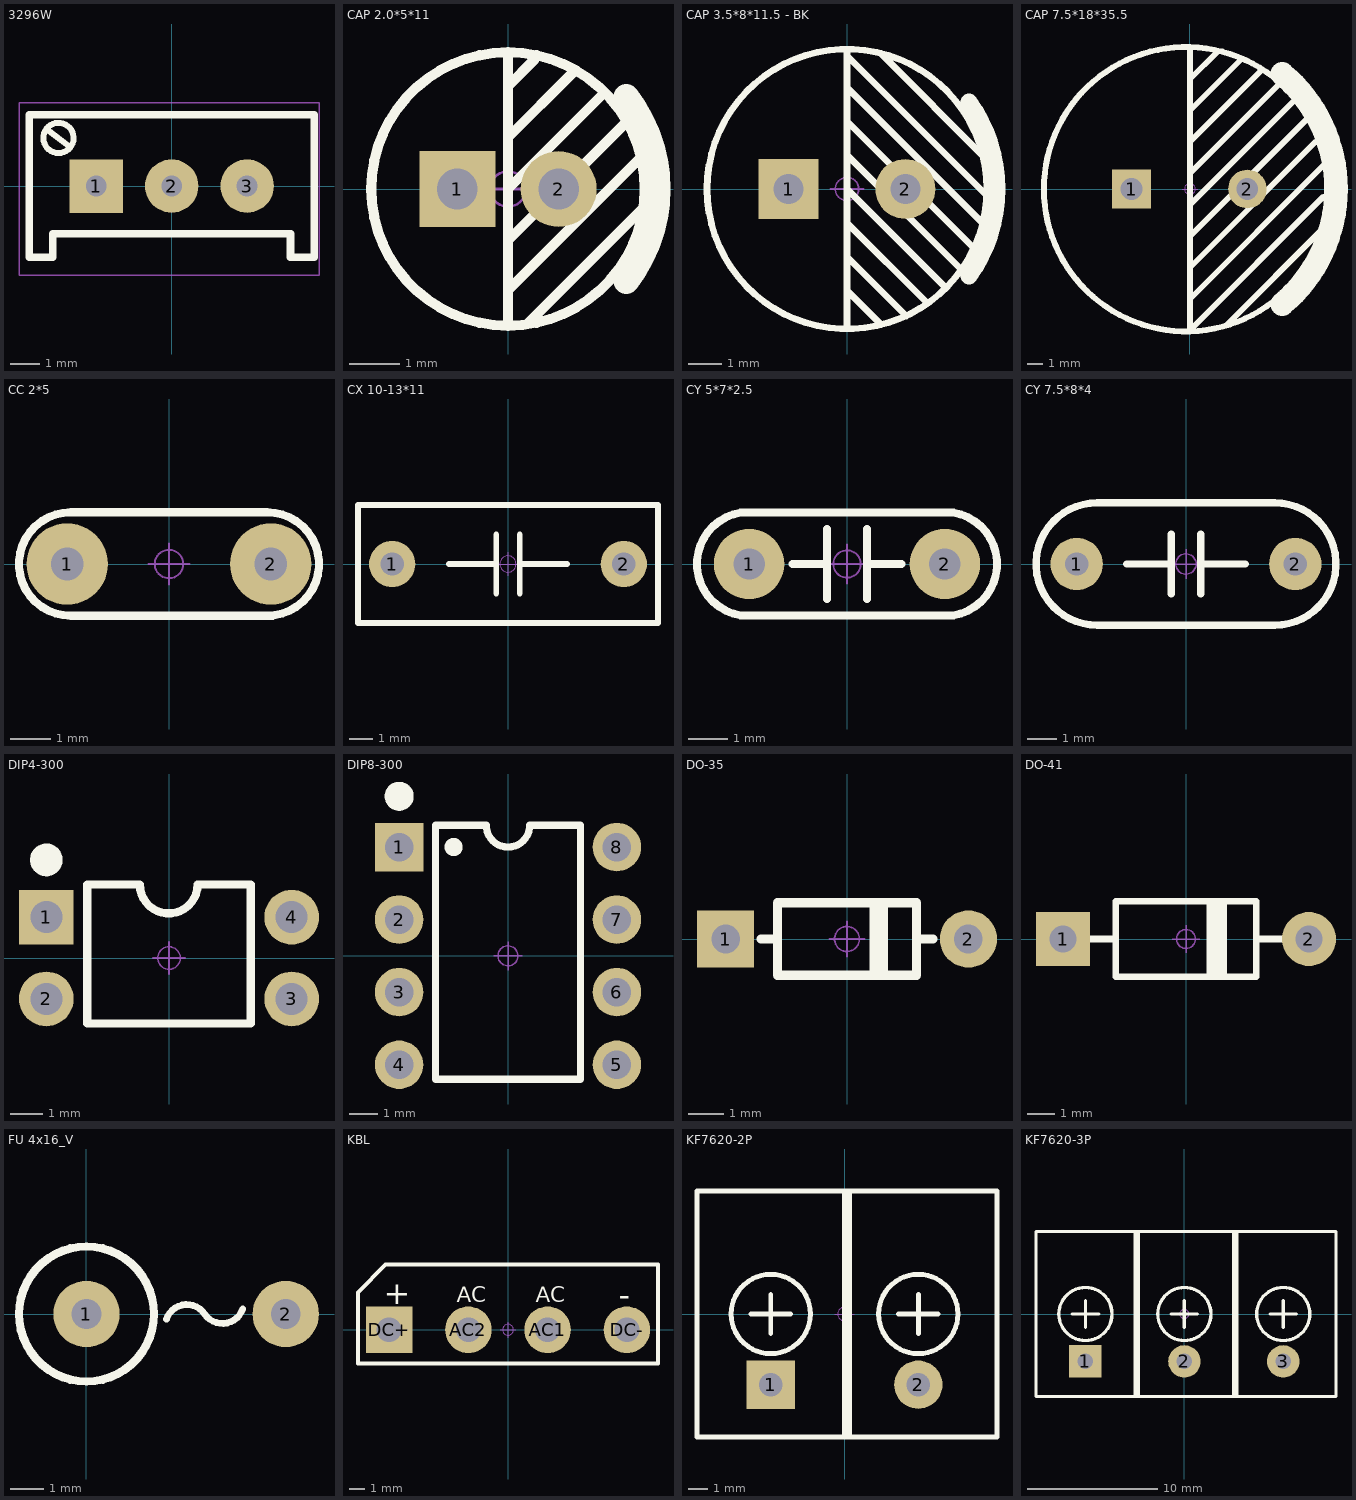
[diagram p0: the footprints below, top view; thin cyan lines are the x and y axes]
# Altium footprint library MISC82119-3.PcbLib: 27 footprints (part 1 of 2)
Each footprint in its own frame and in the unit in brackets; x right, y up, seen from the top. Pads: shape width x height; smd on the part's side, far side on the other; paste and mask are expansions set on the pad; w line width, h text height; cw(c..) or ccw(c..) is an arc to the next point about the centre after c.

## 3296W [mm] "Precise Multi-Winding Adjustable Resistor"
height 6.35
pads (3):
  rect 1.8x1.8 hole 0.7: 1(-2.54,0)
  round 1.8 hole 0.7: 2(0,0) 3(2.54,0)
Top Overlay:
  lines w0.2: -3.302,1.651 ccw(c-3.81,1.618) -3.301,1.608
  lines w0.203: -4.2,1.9 -3.464,1.348
  lines w0.254: -4.8,-2.4 -4,-2.4 -4,-1.6 4,-1.6 4,-2.4 4.8,-2.4 4.8,2.4 -4.8,2.4 -4.8,-2.4
Mechanical 15:
  lines w0.05: -5.14,-3 -5.14,2.8 4.96,2.8 4.96,-3 -5.14,-3
3D body "3296.STEP": height 11.52, standoff -3.48, extent -4.75,-2.4 4.75,2.4

## CAP 2.0*5*11 [mm]
pads (2):
  rect 1.5x1.5 hole 0.8: 1(-1,0)
  round 1.5 hole 0.8: 2(1,0)
Top Overlay:
  circle w0.2: c0,0 r2.7
  lines w0.2: 0,-2.667 0,-2 ; 0,-1.016 2.286,1.27 ; 0,0 1.905,1.905 ; 0,1.016 1.27,2.286 ; 0,2.032 0.508,2.54 ; 0,2.667 0,-2 ; 0.381,-2.667 2.667,-0.381 ; 2.651,0.651 0,-2
  lines w0.5: 2.338,-1.819 ccw(c0,0) 2.338,1.819
Mechanical 15:
  circle w0.05: c0,0 r0.35
  lines w0.05: -0.5,0 0.5,0 ; 0,-0.5 0,0.5
3D body "CAP 2X5X11.STEP": height 11.04, standoff -3.42, extent -2.5,-2.499 2.51,2.499

## CAP 3.5*8*11.5 - BK [mm] "Pin pitch 3.5mm, diameter 8mm, height 11.5mm"
pads (2):
  rect 1.8x1.8 hole 0.9: 1(-1.75,0)
  round 1.8 hole 0.9: 2(1.75,0)
Top Overlay:
  circle w0.2: c0,0 r4.2
  lines w0.2: 0,-4.191 0,4 ; 0,-3.048 1.016,-4.064 ; 0,-2.032 1.778,-3.81 ; 0,-1.016 2.413,-3.429 ; 0,0 2.921,-2.921 ; 0,1.016 3.429,-2.413 ; 0,2.032 3.81,-1.778 ; 0,3.048 4.064,-1.016 ; 0,4.191 0,4 ; 1.016,4.064 4.191,0.889 ; 4.191,-0.127 4.127,-0.127 0,4
  lines w0.504: 3.663,-2.616 ccw(c0,0) 3.663,2.616
Mechanical 15:
  circle w0.05: c0,0 r0.35
  lines w0.05: -0.5,0 0.5,0 ; 0,-0.5 0,0.5
3D body "CAP 3.5X8X11.5.STEP": height 11.54, standoff -3.37, extent -4,-4 4.01,4

## CAP 7.5*18*35.5 [mm]
height 6.35
pads (2):
  rect 2.5x2.5 hole 1.4: 1(-3.78,0)
  round 2.5 hole 1.4: 2(3.72,0)
Top Overlay:
  circle w0.381: c-0.248,-0.013 r9.2
  lines w0.381: 0,-7.112 8.636,1.524 ; 0,-5.08 8.128,3.048 ; 0,-3.048 7.62,4.572 ; 0,-1.016 6.731,5.715 ; 0,1.016 5.715,6.731 ; 0,3.048 4.572,7.62 ; 0,5.08 3.302,8.382 ; 0,7.112 1.778,8.89 ; 0,9.144 0,-9.144 8.636,-0.508 ; 2.413,-8.763 8.636,-2.54
  lines w1.524: 5.959,-7.456 ccw(c-0.254,0) 5.959,7.456
Mechanical 15:
  circle w0.05: c0,0 r0.35
  lines w0.05: -0.5,0 0.5,0 ; 0,-0.5 0,0.5
3D body "CAP 7.5X18X35.5.STEP": height 35.54, standoff -3.37, extent -9,-8.997 9.01,8.997

## CC 2*5 [mm] "Pin pitch 2.2mm, diameter 5mm"
height 6.35
pads (2):
  round 2 hole 0.8: 1(-2.5,0) 2(2.5,0)
Top Overlay:
  lines w0.2: -2.413,1.27 2.413,1.27 ; -2.413,1.271 ccw(c-2.413,0.001) -2.413,-1.27 2.54,-1.27 ; 2.413,-1.27 ccw(c2.413,0.001) 2.413,1.271
Mechanical 15:
  circle w0.05: c0,0 r0.35
  lines w0.05: -0.5,0 0.5,0 ; 0,-0.5 0,0.5
3D body "CC 2.2X5.STEP": height 4.8, standoff -3.5, extent -2.4,-0.917 2.4,0.918

## CX 10-13*11 [mm]
pads (2):
  round 2 hole 1: 1(-5,0) 2(5,0)
Top Overlay:
  lines w0.254: -2.54,0 -0.604,0 ; -0.508,-1.27 -0.508,1.27 ; 0.508,-1.27 0.508,1.27 ; 0.508,0 2.54,0 ; -6.477,-2.54 4.953,-2.54 6.477,-2.54 6.477,2.54 4.953,2.54 -6.477,2.54 -6.477,-2.54
Mechanical 15:
  circle w0.05: c0,0 r0.35
  lines w0.05: -0.5,0 0.5,0 ; 0,-0.5 0,0.5
3D body "CX 10X13X11.STEP": height 11.02, standoff -3.48, extent -6.5,-2.5 6.5,2.5

## CY 5*7*2.5 [mm]
pads (2):
  round 1.8 hole 0.8: 1(-2.5,0) 2(2.5,0)
Top Overlay:
  lines w0.203: -1.397,0 -0.508,0 ; -0.508,-0.889 -0.508,0.889 ; 0.508,-0.889 0.508,0.889 ; 0.508,0 1.397,0 ; -2.726,1.313 ccw(c-2.5,0) -2.726,-1.313 2.726,-1.313 2.726,-1.313 ccw(c2.5,0) 2.726,1.313 -2.726,1.313 -2.726,1.313
Mechanical 15:
  circle w0.05: c0,0 r0.35
  lines w0.05: -0.5,0 0.5,0 ; 0,-0.5 0,0.5
3D body "CY 5X7X2.5.STEP": height 7, standoff -3.5, extent -3.5,-1.25 3.5,1.25

## CY 7.5*8*4 [mm] "Pin pitch 7.5mm, diameter 8mm, thickness 4mm"
height 6.35
pads (2):
  round 1.8 hole 0.8: 1(-3.75,0) 2(3.75,0)
Top Overlay:
  lines w0.254: -2.032,0 -0.508,0 ; -0.508,-1.016 -0.508,1.016 ; 0.508,-1.016 0.508,1.016 ; 0.508,0 2.032,0 ; -3.048,-2.1 cw(c-3.048,0) -3.048,2.1 3.048,2.1 cw(c3.048,0) 3.048,-2.1 -3.048,-2.1
Mechanical 15:
  circle w0.05: c0,0 r0.35
  lines w0.05: -0.5,0 0.5,0 ; 0,-0.5 0,0.5
3D body "CY 7.5X8X4.STEP": height 8.2, standoff -3.3, extent -4.042,-2 4.042,2

## DIP4-300 [mm]
pads (4):
  rect 1.7x1.7 hole 1: 1(-3.81,1.27)
  round 1.7 hole 1: 2(-3.81,-1.27) 3(3.81,-1.27) 4(3.81,1.27)
Top Overlay:
  circle w0.508: c-3.81,3.048 r0.254
  lines w0.254: -2.54,-2.032 2.54,-2.032 2.54,2.286 0.889,2.286 cw(c-0.009,2.286) -0.907,2.286 -2.54,2.286 -2.54,-2.032
Mechanical 15:
  circle w0.05: c0,0 r0.35
  lines w0.05: -0.5,0 0.5,0 ; 0,-0.5 0,0.5
3D body "DIP4-300.STEP": height 4.5, standoff -3.29, extent -3.935,-2.29 3.935,2.29

## DIP8-300 [mm]
pads (8):
  rect 1.7x1.7 hole 1: 1(-3.81,3.81)
  round 1.7 hole 1: 2(-3.81,1.27) 3(-3.81,-1.27) 4(-3.81,-3.81) 5(3.81,-3.81) 6(3.81,-1.27) 7(3.81,1.27) 8(3.81,3.81)
Top Overlay:
  circle w0.381: c-1.905,3.81 r0.127
  circle w0.508: c-3.81,5.588 r0.254
  lines w0.254: -2.54,-4.318 -2.54,4.572 -0.762,4.572 ccw(c0,4.572) 0,3.81 ccw(c0,4.572) 0.762,4.572 2.54,4.572 2.54,-4.318 -2.54,-4.318
Mechanical 15:
  circle w0.05: c0,0 r0.35
  lines w0.05: -0.5,0 0.5,0 ; 0,-0.5 0,0.5
3D body "DIP8-300.STEP": height 4.5, standoff -3.2, extent -3.925,-4.7 3.925,4.7

## DO-35 [mm]
pads (2):
  rect 1.6x1.6 hole 0.8: 1(-3.4,0)
  round 1.6 hole 0.8: 2(3.4,0)
Top Overlay:
  rectangle: 0.635,-1.016 1.143,1.016
  lines w0.254: -2.413,0 -1.95,0 ; 1.95,0 2.413,0 ; -1.95,-1.016 -1.95,1.016 1.95,1.016 1.95,-1.016 -1.95,-1.016
Mechanical 15:
  circle w0.05: c0,0 r0.35
  lines w0.05: -0.5,0 0.5,0 ; 0,-0.5 0,0.5
3D body "DO-35.STEP": height 1.85, standoff -3.45, extent -3.65,-0.901 3.65,0.901

## DO-41 [mm]
height 2.4
pads (2):
  rect 2x2 hole 1: 1(-4.55,0)
  round 2 hole 1: 2(4.55,0)
Top Overlay:
  rectangle: 0.762,-1.397 1.524,1.397
  lines w0.254: -3.556,0 -2.6,0 ; 2.6,0 3.556,0 ; -2.6,-1.397 -2.6,1.397 2.6,1.397 2.6,-1.397 -2.6,-1.397
Mechanical 15:
  circle w0.05: c0,0 r0.35
  lines w0.05: -0.5,0 0.5,0 ; 0,-0.5 0,0.5
3D body "DO-41.STEP": height 2.65, standoff -3.45, extent -4.925,-1.288 4.975,1.314

## FU 4x16_V [mm]
pads (2):
  round 2 hole 0.9: 1(0,0) 2(6,0)
Top Overlay:
  circle w0.254: c0,0 r2.032
  lines w0.203: 2.406,-0.156 cw(c3.019,-0.362) 3.556,0 ccw(c4.093,0.362) 4.706,0.156
3D body "FU 4x16_V.STEP": height 13.1, standoff -3.55, extent -2,-2 6.3,2

## KBL [mm]
pads (4):
  round 3 hole 1.6: AC1(2.55,0) AC2(-2.55,0) DC-(7.65,0)
  rect 3x3 hole 1.6: DC+(-7.65,0)
Top Overlay:
  lines w0.254: -9.652,-2.159 9.652,-2.159 9.652,4.191 -7.874,4.191 -9.652,2.413 -9.652,-2.159
  text "AC" at 1.778,1.778 h1
  text "AC" at -3.302,1.778 h1
  text "-" at 7.112,1.524 h1.5
  text "+" at -8.001,1.651 h1.5
Mechanical 15:
  circle w0.05: c0,0 r0.35
  lines w0.05: -0.5,0 0.5,0 ; 0,-0.5 0,0.5
3D body "KBL.STEP": height 14.21, standoff -3.49, extent -9.5,-2.1 9.5,4.15

## KF7620-2P [mm] "15.2*12*12mm (L*W*H)"
pads (2):
  rect 2.5x2.5 hole 1.2: 1(-3.81,-3.65)
  round 2.5 hole 1.2: 2(3.81,-3.65)
Top Overlay:
  circle w0.254: c3.81,0 r2.048
  circle w0.254: c-3.81,0 r2.048
  lines w0.254: -4.826,0 -2.794,0 ; -3.81,-1.016 -3.81,1.016 ; 0,-6.35 0,6.35 ; 0.254,6.35 0.254,-6.35 0.508,-6.35 ; 2.794,0 4.826,0 ; 3.81,-1.016 3.81,1.016 ; -7.62,-6.35 -7.62,6.35 7.874,6.35 7.874,-6.35 -7.62,-6.35
Mechanical 15:
  circle w0.05: c0,0 r0.35
  lines w0.05: -0.5,0 0.5,0 ; 0,-0.5 0,0.5
3D body "KF7620.STEP": height 12.45, standoff -3.45, extent -7.62,-6.2 0.7,6.2
3D body "KF7620.STEP": height 12.45, standoff -3.45, extent 0,-6.2 8.32,6.2

## KF7620-3P [mm] "22.8*12*12mm (L*W*H)"
pads (3):
  rect 2.5x2.5 hole 1.2: 1(-7.62,-3.65)
  round 2.5 hole 1.2: 2(0,-3.65) 3(7.62,-3.65)
Top Overlay:
  circle w0.254: c7.62,0 r2.048
  circle w0.254: c0,0 r2.048
  circle w0.254: c-7.62,0 r2.048
  lines w0.254: -8.636,0 -6.604,0 ; -7.62,-1.016 -7.62,1.016 ; -3.81,-6.35 -3.81,6.35 ; -3.556,6.35 -3.556,-6.35 -3.302,-6.35 ; -1.016,0 1.016,0 ; 0,-1.016 0,1.016 ; 3.81,-6.35 3.81,6.35 ; 6.604,0 8.636,0 ; 7.62,-1.016 7.62,1.016 ; 4.064,-6.35 11.684,-6.35 11.684,6.35 4.064,6.35 ; 4.064,-6.35 -11.43,-6.35 -11.43,6.35 4.064,6.35 ; 4.064,-6.35 4.064,6.35
Mechanical 15:
  circle w0.05: c0,0 r0.35
  lines w0.05: -0.5,0 0.5,0 ; 0,-0.5 0,0.5
3D body "KF7620.STEP": height 12.45, standoff -3.45, extent 3.81,-6.2 12.13,6.2
3D body "KF7620.STEP": height 12.45, standoff -3.45, extent -11.43,-6.2 -3.11,6.2
3D body "KF7620.STEP": height 12.45, standoff -3.45, extent -3.81,-6.2 4.51,6.2